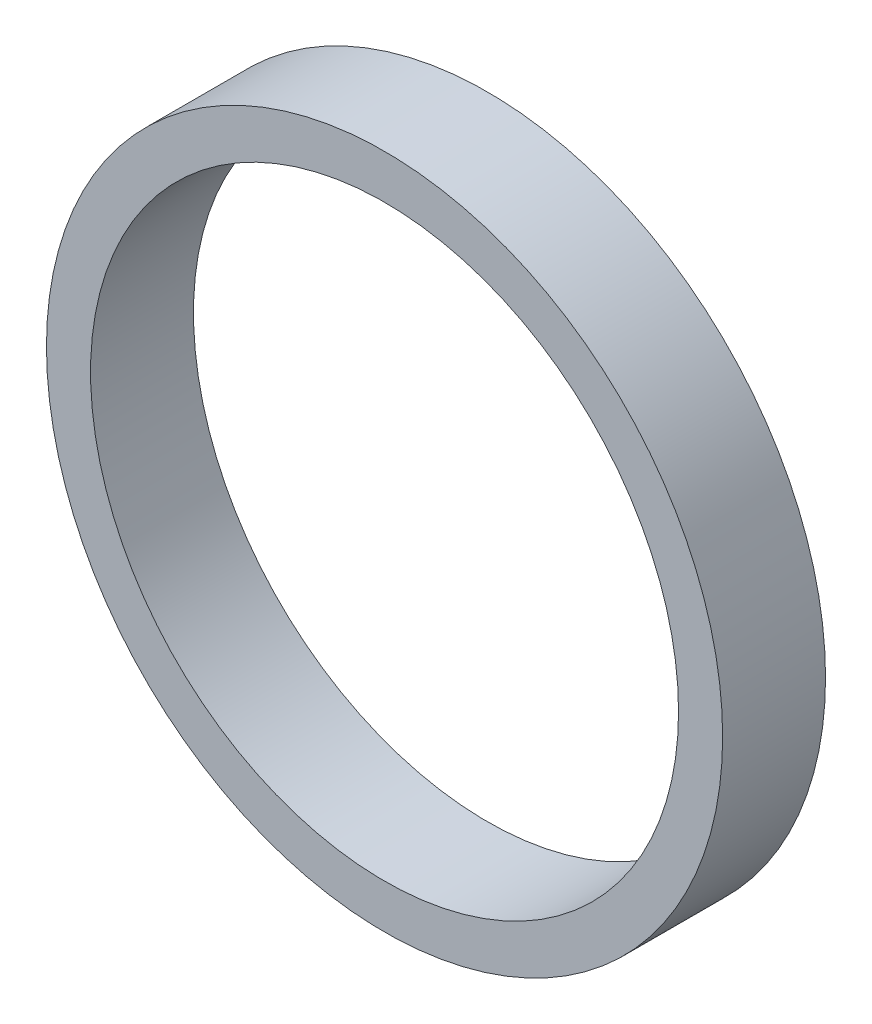
from build123d import *

# Parameters (mm, degrees)
SKETCH_1_R      = 23
SKETCH_1_R_2    = 20
EXTRUDE_1_DEPTH = 7


with BuildPart() as part:
    # 草图1 → 凸台-拉伸1 (new body)
    with BuildSketch(Plane.XY):
        Circle(SKETCH_1_R)
        Circle(SKETCH_1_R_2, mode=Mode.SUBTRACT)
    extrude(amount=EXTRUDE_1_DEPTH)


solid = part.part
